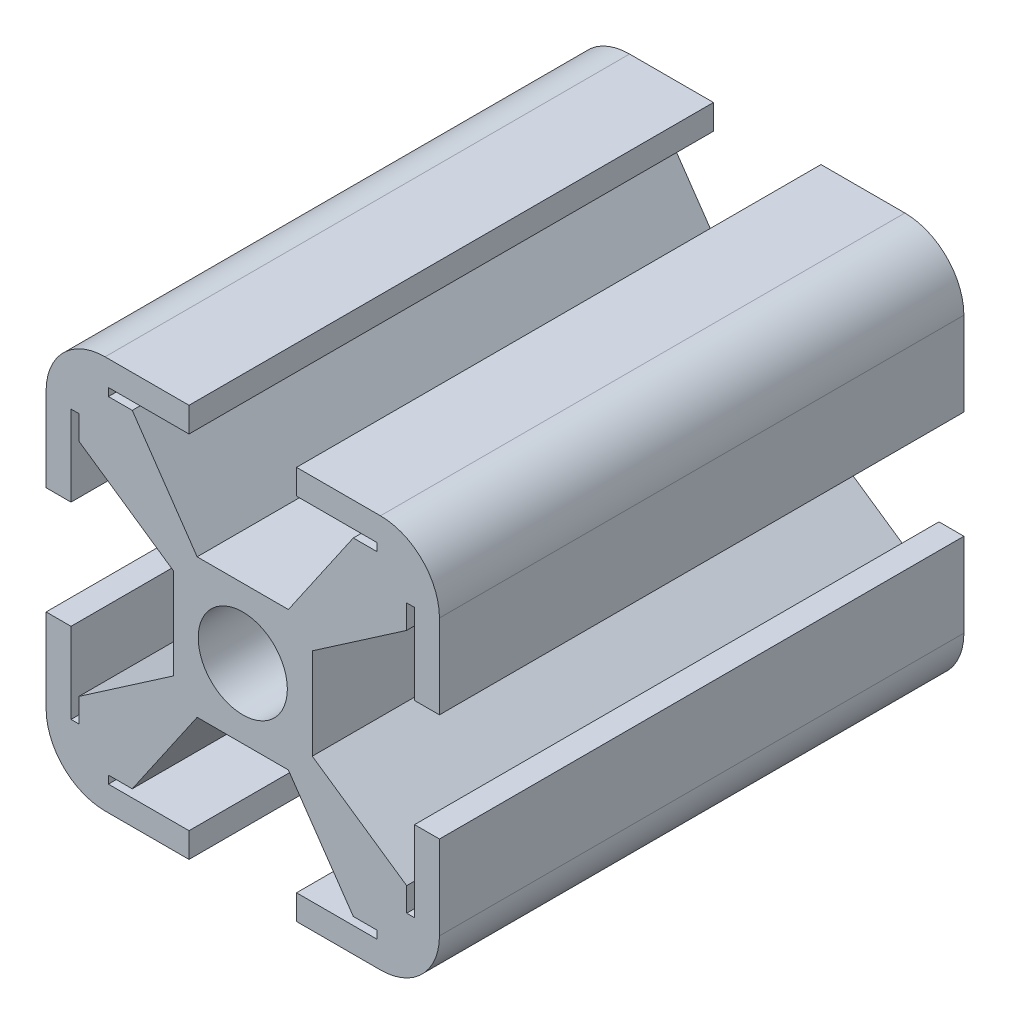
from build123d import *

# Parameters (mm, degrees)
SKETCH_1_W               = 30
SKETCH_1_H               = 30
EXTRUDE_1_DEPTH          = 20
FILLET_1_R               = 4.5
SKETCH_2_W               = 8.2
SKETCH_2_H               = 0.3
SKETCH_2_H_2             = 1.9
SKETCH_2_R               = 3.4
CUT_EXTRUDE_1_DEPTH      = 46.276925691
PATTERN_CIRCULAR_1_COUNT = 4


with BuildPart() as part:
    # 草图1 → 凸台-拉伸1 (new, symmetric)
    with BuildSketch(Plane.XY):
        Rectangle(SKETCH_1_W, SKETCH_1_H)
    extrude(amount=EXTRUDE_1_DEPTH, both=True)

    # 圆角1
    fillet_1_edges = [part.edges().sort_by_distance(p)[0] for p in [
        (-15, 15, 0),
        (15, 15, 0),
        (15, -15, 0),
        (-15, -15, 0),
    ]]
    fillet(fillet_1_edges, radius=FILLET_1_R)

    # 草图2 → 切除-拉伸1 (cut, through all)
    with BuildSketch(Plane.XY.offset(20)):
        with Locations((0, 12.95)):
            Rectangle(SKETCH_2_W, SKETCH_2_H)
        with Locations((0, 14.05)):
            Rectangle(SKETCH_2_W, SKETCH_2_H_2)
        Polygon((10.25, 13.1), (4.1, 13.1), (4.1, 12.8), (-4.1, 12.8), (-4.1, 13.1), (-10.25, 13.1), (-10.25, 12.5), (-8.429704265, 12.5), (8.429704265, 12.5), (10.25, 12.5), align=None)
        Polygon((3.479704265, 5.3), (8.429704265, 12.5), (-8.429704265, 12.5), (-3.479704265, 5.3), align=None)
        Circle(SKETCH_2_R)
    cut_extrude_1 = extrude(amount=-CUT_EXTRUDE_1_DEPTH, mode=Mode.SUBTRACT)

    # 阵列(圆周)1: 切除-拉伸1 ×4 about axis
    pattern_circular_1_axis = Axis((0, 0, 0), (0, 0, 1))
    for i in range(1, PATTERN_CIRCULAR_1_COUNT):
        add(cut_extrude_1.rotate(pattern_circular_1_axis, i * 360 / PATTERN_CIRCULAR_1_COUNT), mode=Mode.SUBTRACT)


solid = part.part
